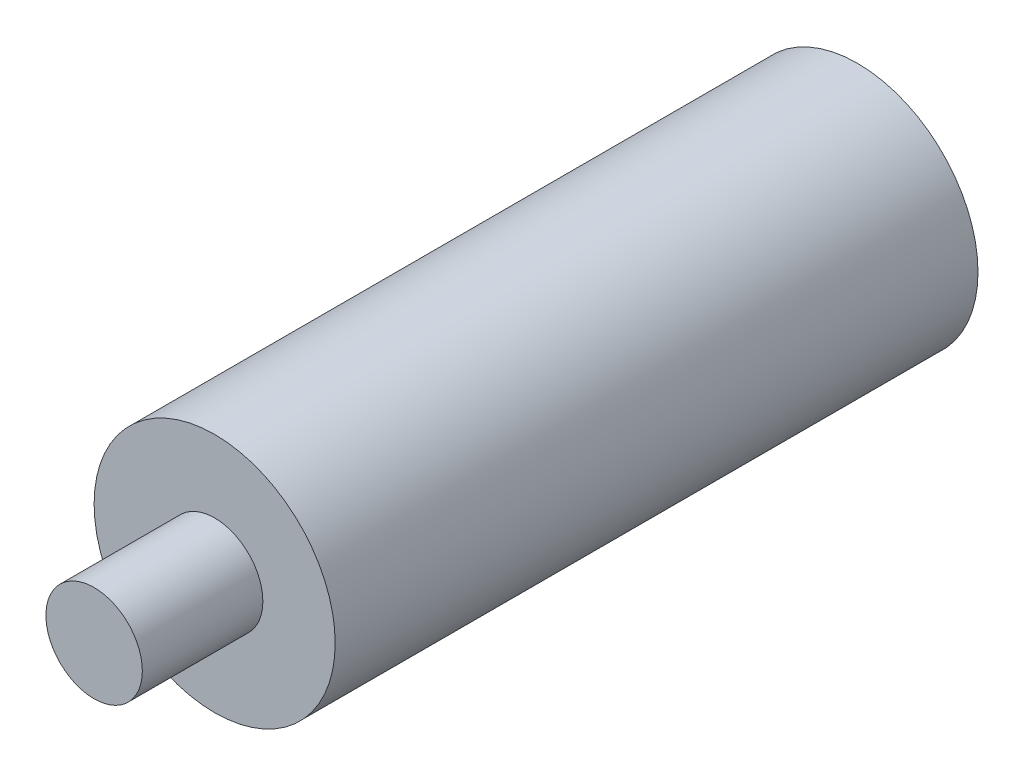
from build123d import *

# Parameters (mm, degrees)
SKETCH_1_R              = 15
EXTRUDE_1_DEPTH         = 40
HOLE_WIZARD_M10_1_D     = 8.5
HOLE_WIZARD_M10_1_DEPTH = 20
HOLE_WIZARD_M10_1_TIP   = 2.553657631
SKETCH_4_R              = 6
EXTRUDE_2_DEPTH         = 15


with BuildPart() as part:
    # 草图1 → 凸台-拉伸1 (new, symmetric)
    with BuildSketch(Plane.XY):
        Circle(SKETCH_1_R)
    extrude(amount=EXTRUDE_1_DEPTH, both=True)

    # M10 螺纹孔1
    with Locations(Plane(origin=(0, 0, -40), x_dir=(-1, 0, 0), z_dir=(0, 0, -1))):
        with Locations((0, 0)):
            Hole(HOLE_WIZARD_M10_1_D / 2, depth=HOLE_WIZARD_M10_1_DEPTH)
            with Locations((0, 0, -(HOLE_WIZARD_M10_1_DEPTH + HOLE_WIZARD_M10_1_TIP / 2))):  # 118° drill point
                Cone(0, HOLE_WIZARD_M10_1_D / 2, HOLE_WIZARD_M10_1_TIP, mode=Mode.SUBTRACT)

    # 草图4 → 凸台-拉伸2 (add)
    with BuildSketch(Plane.XY.offset(40)):
        Circle(SKETCH_4_R)
    extrude(amount=EXTRUDE_2_DEPTH)


solid = part.part
